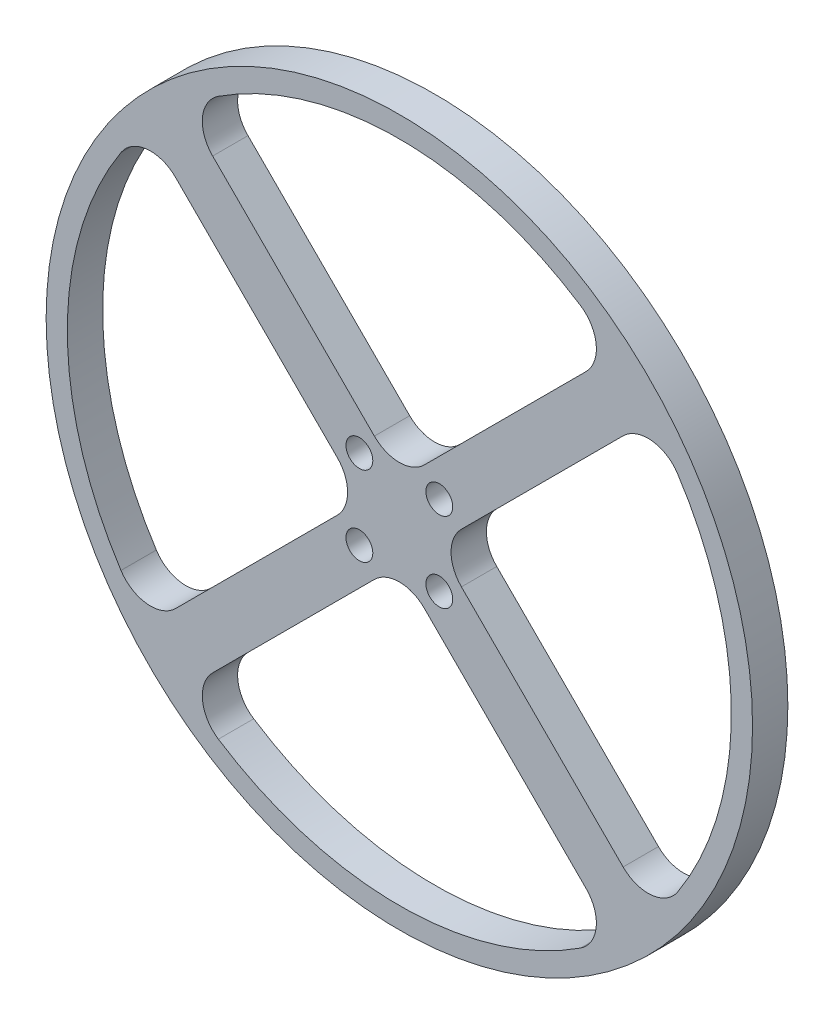
SolidWorks part; units mm, degrees
material "Acrylic (Medium-high impact)"
ref_plane "Front Plane" through (0, 0, 0) normal (0, 0, 1) x (1, 0, 0)
ref_plane "Top Plane" through (0, 0, 0) normal (0, 1, 0) x (1, 0, 0)
ref_plane "Right Plane" through (0, 0, 0) normal (1, 0, 0) x (0, 0, -1)
sketch "Sketch1" plane through (0, 0, 0) normal (0, 0, 1) x (1, 0, 0)
  line L0 (30.5045, 35.7558) -> (0, 5.2513)
  line L2 (5.2513, 0) -> (35.7558, 30.5045)
  line L3 (0, 0) -> (28.2843, 28.2843) construction
  line L4 (5.2513, 0) -> (35.7558, -30.5045)
  line L5 (0, -5.2513) -> (30.5045, -35.7558)
  line L6 (0, -5.2513) -> (-30.5045, -35.7558)
  line L7 (-5.2513, 0) -> (-35.7558, -30.5045)
  line L8 (-5.2513, 0) -> (-35.7558, 30.5045)
  line L9 (-30.5045, 35.7558) -> (0, 5.2513)
  line L10 (0, 0) -> (13.7365, -13.7365) construction
  circle A1 centre (0, 0) radius 50
  arc A2 (30.5045, 35.7558) -> (-30.5045, 35.7558) centre (0, 0) ccw
  arc A8 (-30.5045, -35.7558) -> (30.5045, -35.7558) centre (0, 0) ccw
  arc A9 (-35.7558, 30.5045) -> (-35.7558, -30.5045) centre (0, 0) ccw
  arc A10 (35.7558, -30.5045) -> (35.7558, 30.5045) centre (0, 0) ccw
  dimension "D1" = 100
  dimension "D2" = 47
  dimension "D3" = 5.2513
extrude "Boss-Extrude1" add sketch "Sketch1" along normal blind 5
fillet "Fillet1" radius 5 12 edges at (30.5045, -35.7558, 2.5) (35.7558, -30.5045, 2.5) (-30.5045, -35.7558, 2.5) (0, -5.2513, 2.5) (5.2513, 0, 2.5) (35.7558, 30.5045, 2.5) (30.5045, 35.7558, 2.5) (-30.5045, 35.7558, 2.5) (-35.7558, 30.5045, 2.5) (0, 5.2513, 2.5) (-5.2513, 0, 2.5) (-35.7558, -30.5045, 2.5)
sketch "Sketch2" plane through (0, 0, 5) normal (0, 0, 1) x (1, 0, 0)
  circle A0 centre (5.6569, -5.6569) radius 1.9 construction
  circle A1 centre (5.6569, 5.6569) radius 1.9 construction
  circle A2 centre (-5.6569, 5.6569) radius 1.9 construction
  circle A3 centre (-5.6569, -5.6569) radius 1.9 construction
  circle A4 centre (5.6569, -5.6569) radius 1.9
  circle A5 centre (5.6569, 5.6569) radius 1.9
  circle A6 centre (-5.6569, 5.6569) radius 1.9
  circle A7 centre (-5.6569, -5.6569) radius 1.9
extrude "Cut-Extrude1" cut sketch "Sketch2" against normal blind 5
